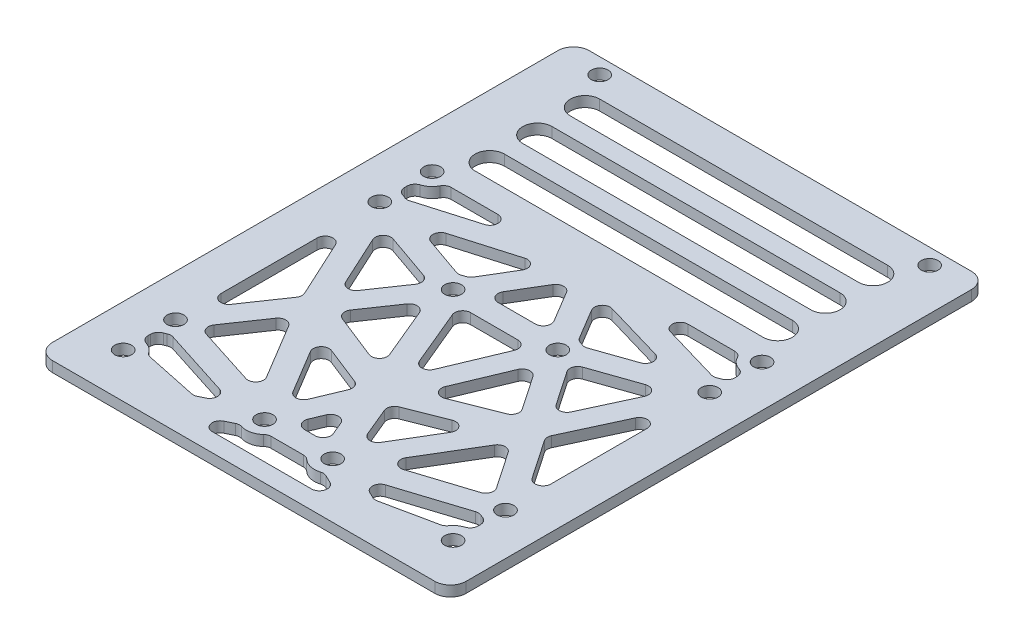
from build123d import *

# Parameters (mm, degrees)
SKETCH_1_W          = 79
SKETCH_1_H          = 102.5
SKETCH_1_R          = 1.6
EXTRUDE_1_DEPTH     = 2
CUT_EXTRUDE_1_DEPTH = 69.558369292
FILLET_R1_5_R       = 1.5
FILLET_R3_R         = 3


with BuildPart() as part:
    # 草图1 → 凸台-拉伸1 (new body)
    with BuildSketch(Plane(origin=(0, 0, 0), x_dir=(1, 0, 0), z_dir=(0, 1, 0))):
        with Locations((0, 4.75)):
            Rectangle(SKETCH_1_W, SKETCH_1_H)
        with Locations(Location((-31.5, 11, 0), (0, 0, 270))):
            Circle(SKETCH_1_R, mode=Mode.SUBTRACT)
        with Locations(Location((-31.5, 21, 0), (0, 0, 270))):
            Circle(SKETCH_1_R, mode=Mode.SUBTRACT)
        with Locations(Location((31.5, 11, 0), (0, 0, 90))):
            Circle(SKETCH_1_R, mode=Mode.SUBTRACT)
        with Locations(Location((31.5, 21, 0), (0, 0, 90))):
            Circle(SKETCH_1_R, mode=Mode.SUBTRACT)
        with Locations(Location((-6.5, -36, 0), (0, 0, 270))):
            Circle(SKETCH_1_R, mode=Mode.SUBTRACT)
        with Locations(Location((6.5, -36, 0), (0, 0, 90))):
            Circle(SKETCH_1_R, mode=Mode.SUBTRACT)
        with Locations(Location((-10, 3.5, 0), (0, 0, 270))):
            Circle(SKETCH_1_R, mode=Mode.SUBTRACT)
        with Locations(Location((10, 3.5, 0), (0, 0, 90))):
            Circle(SKETCH_1_R, mode=Mode.SUBTRACT)
        with Locations(Location((-31.5, 53, 0), (0, 0, 270))):
            Circle(SKETCH_1_R, mode=Mode.SUBTRACT)
        with Locations(Location((31.5, 53, 0), (0, 0, 90))):
            Circle(SKETCH_1_R, mode=Mode.SUBTRACT)
        with Locations(Location((-31.5, -28, 0), (0, 0, 270))):
            Circle(SKETCH_1_R, mode=Mode.SUBTRACT)
        with Locations(Location((-31.5, -38, 0), (0, 0, 270))):
            Circle(SKETCH_1_R, mode=Mode.SUBTRACT)
        with Locations(Location((31.5, -38, 0), (0, 0, 90))):
            Circle(SKETCH_1_R, mode=Mode.SUBTRACT)
        with Locations(Location((31.5, -28, 0), (0, 0, 90))):
            Circle(SKETCH_1_R, mode=Mode.SUBTRACT)
    extrude(amount=EXTRUDE_1_DEPTH)

    # 草图2 → 切除-拉伸1 (cut, through all)
    with BuildSketch(Plane(origin=(0, 2, 0), x_dir=(1, 0, 0), z_dir=(0, 1, 0))):
        with BuildLine():
            Line((-27.5, 43.4), (27.5, 43.4))
            ThreePointArc((27.5, 43.4), (30.3, 46.2), (27.5, 49))
            Line((27.5, 49), (-27.5, 49))
            ThreePointArc((-27.5, 49), (-30.3, 46.2), (-27.5, 43.4))
        make_face()
        with BuildLine():
            Line((-27.5, 34.3), (27.5, 34.3))
            ThreePointArc((27.5, 34.3), (30.3, 37.1), (27.5, 39.9))
            Line((27.5, 39.9), (-27.5, 39.9))
            ThreePointArc((-27.5, 39.9), (-30.3, 37.1), (-27.5, 34.3))
        make_face()
        with BuildLine():
            Line((-27.5, 25.2), (27.5, 25.2))
            ThreePointArc((27.5, 25.2), (30.3, 28), (27.5, 30.8))
            Line((27.5, 30.8), (-27.5, 30.8))
            ThreePointArc((-27.5, 30.8), (-30.3, 28), (-27.5, 25.2))
        make_face()
        with BuildLine():
            Line((-31.5, 17.5), (-31.5, 14.5))
            ThreePointArc((-31.5, 14.5), (-30.423705251, 14.330403821), (-29.451716488, 13.838051207))
            Line((-29.451716488, 13.838051207), (-7.668957034, 20.2))
            Line((-7.668957034, 20.2), (-28.092654993, 20.2))
            ThreePointArc((-28.092654993, 20.2), (-29.326293488, 18.256826655), (-31.5, 17.5))
        make_face()
        with BuildLine():
            ThreePointArc((29.451716488, 13.838051207), (30.423705251, 14.330403821), (31.5, 14.5))
            Line((31.5, 14.5), (31.5, 17.5))
            ThreePointArc((31.5, 17.5), (29.326293488, 18.256826655), (28.092654993, 20.2))
            Line((28.092654993, 20.2), (7.668957034, 20.2))
            Line((7.668957034, 20.2), (29.451716488, 13.838051207))
        make_face()
        with BuildLine():
            Line((-24.452290628, 10.818556238), (-11.899535217, 6.439688072))
            ThreePointArc((-11.899535217, 6.439688072), (-11.192938065, 6.790425318), (-10.425740034, 6.974009992))
            Line((-10.425740034, 6.974009992), (-4.662637344, 16.598391483))
            Line((-4.662637344, 16.598391483), (-24.452290628, 10.818556238))
        make_face()
        Polygon((-6.206589312, 5.65), (6.206589312, 5.65), (0, 16.015004152), align=None)
        with BuildLine():
            Line((11.899535217, 6.439688072), (24.452290628, 10.818556238))
            Line((24.452290628, 10.818556238), (4.662637344, 16.598391483))
            Line((4.662637344, 16.598391483), (10.425740034, 6.974009992))
            ThreePointArc((10.425740034, 6.974009992), (11.192938065, 6.790425318), (11.899535217, 6.439688072))
        make_face()
        Polygon((-27.420486956, 7.299854547), (-20.389131694, -7.907495205), (-13.357776432, 2.394257853), align=None)
        Polygon((-17.456513392, -11.238449922), (-3.946122396, -16.570590362), (-10.457154201, -0.983574828), align=None)
        Polygon((-6.771858845, 1.35), (0, -14.86141966), (6.771858845, 1.35), align=None)
        Polygon((-31.5, 5.87701259), (-31.5, -24.186209235), (-23.213342702, -12.045292729), align=None)
        Polygon((13.357776432, 2.394257853), (20.389131694, -7.907495205), (27.420486956, 7.299854547), align=None)
        Polygon((10.457154201, -0.983574828), (3.946122396, -16.570590362), (17.456513392, -11.238449922), align=None)
        Polygon((23.213342702, -12.045292729), (31.5, -24.186209235), (31.5, 5.87701259), align=None)
        Polygon((-28.098995565, -26.830923802), (-11.279390947, -32.21319728), (-20.866565579, -16.234572893), align=None)
        Polygon((-15.647599969, -16.575151194), (-6.844560738, -31.246883245), (-2.829139335, -21.634207764), align=None)
        Polygon((-3.271858845, -33.85), (3.271858845, -33.85), (0, -26.017368219), align=None)
        Polygon((2.829139335, -21.634207764), (6.844560738, -31.246883245), (15.647599969, -16.575151194), align=None)
        Polygon((20.866565579, -16.234572893), (11.279390947, -32.21319728), (28.098995565, -26.830923802), align=None)
        with BuildLine():
            Line((-28.354506597, -36.465115232), (-17.21554823, -38.810303281))
            Line((-17.21554823, -38.810303281), (-12.270862978, -36.410721464))
            Line((-12.270862978, -36.410721464), (-29.52486957, -30.889439354))
            ThreePointArc((-29.52486957, -30.889439354), (-30.466326391, -31.343877819), (-31.5, -31.5))
            Line((-31.5, -31.5), (-31.5, -34.5))
            ThreePointArc((-31.5, -34.5), (-29.645558937, -35.031658991), (-28.354506597, -36.465115232))
        make_face()
        with BuildLine():
            Line((-8.046002547, -39.140043969), (-16, -43))
            Line((-16, -43), (16, -43))
            Line((16, -43), (8.046002547, -39.140043969))
            ThreePointArc((8.046002547, -39.140043969), (5.716046361, -39.41107266), (3.738207104, -38.15))
            Line((3.738207104, -38.15), (-3.738207104, -38.15))
            ThreePointArc((-3.738207104, -38.15), (-5.716046361, -39.41107266), (-8.046002547, -39.140043969))
        make_face()
        with BuildLine():
            Line((12.270862978, -36.410721464), (17.21554823, -38.810303281))
            Line((17.21554823, -38.810303281), (28.354506597, -36.465115232))
            ThreePointArc((28.354506597, -36.465115232), (29.645558937, -35.031658991), (31.5, -34.5))
            Line((31.5, -34.5), (31.5, -31.5))
            ThreePointArc((31.5, -31.5), (30.466326391, -31.343877819), (29.52486957, -30.889439354))
            Line((29.52486957, -30.889439354), (12.270862978, -36.410721464))
        make_face()
    extrude(amount=-CUT_EXTRUDE_1_DEPTH, mode=Mode.SUBTRACT)

    # R1.5 镂空圆角
    fillet_r1_5_edges = [part.edges().sort_by_distance(p)[0] for p in [
        (-28.354506597, 1, 36.465115232),
        (-31.5, 1, 34.5),
        (-31.5, 1, 31.5),
        (-29.52486957, 1, 30.889439354),
        (-12.270862978, 1, 36.410721464),
        (-17.21554823, 1, 38.810303281),
        (28.098995565, 1, 26.830923802),
        (11.279390947, 1, 32.21319728),
        (20.866565579, 1, 16.234572893),
        (-3.271858845, 1, 33.85),
        (0, 1, 26.017368219),
        (3.271858845, 1, 33.85),
        (15.647599969, 1, 16.575151194),
        (6.844560738, 1, 31.246883245),
        (2.829139335, 1, 21.634207764),
        (28.354506597, 1, 36.465115232),
        (17.21554823, 1, 38.810303281),
        (12.270862978, 1, 36.410721464),
        (29.52486957, 1, 30.889439354),
        (31.5, 1, 31.5),
        (31.5, 1, 34.5),
        (8.046002547, 1, 39.140043969),
        (16, 1, 43),
        (-16, 1, 43),
        (-8.046002547, 1, 39.140043969),
        (-3.738207104, 1, 38.15),
        (3.738207104, 1, 38.15),
        (6.206589312, 1, -5.65),
        (-6.206589312, 1, -5.65),
        (0, 1, -16.015004152),
        (-10.425740034, 1, -6.974009992),
        (-11.899535217, 1, -6.439688072),
        (-24.452290628, 1, -10.818556238),
        (-4.662637344, 1, -16.598391483),
        (10.425740034, 1, -6.974009992),
        (4.662637344, 1, -16.598391483),
        (24.452290628, 1, -10.818556238),
        (11.899535217, 1, -6.439688072),
        (-27.420486956, 1, -7.299854547),
        (-13.357776432, 1, -2.394257853),
        (-20.389131694, 1, 7.907495205),
        (28.092654993, 1, -20.2),
        (31.5, 1, -17.5),
        (31.5, 1, -14.5),
        (29.451716488, 1, -13.838051207),
        (7.668957034, 1, -20.2),
        (-31.5, 1, -17.5),
        (-28.092654993, 1, -20.2),
        (-7.668957034, 1, -20.2),
        (-29.451716488, 1, -13.838051207),
        (-31.5, 1, -14.5),
        (-20.866565579, 1, 16.234572893),
        (-11.279390947, 1, 32.21319728),
        (-28.098995565, 1, 26.830923802),
        (-15.647599969, 1, 16.575151194),
        (-2.829139335, 1, 21.634207764),
        (-6.844560738, 1, 31.246883245),
        (31.5, 1, -5.87701259),
        (31.5, 1, 24.186209235),
        (23.213342702, 1, 12.045292729),
        (17.456513392, 1, 11.238449922),
        (3.946122396, 1, 16.570590362),
        (10.457154201, 1, 0.983574828),
        (0, 1, 14.86141966),
        (-6.771858845, 1, -1.35),
        (6.771858845, 1, -1.35),
        (-17.456513392, 1, 11.238449922),
        (-10.457154201, 1, 0.983574828),
        (-3.946122396, 1, 16.570590362),
        (-31.5, 1, -5.87701259),
        (-23.213342702, 1, 12.045292729),
        (-31.5, 1, 24.186209235),
        (27.420486956, 1, -7.299854547),
        (20.389131694, 1, 7.907495205),
        (13.357776432, 1, -2.394257853),
    ]]
    fillet(fillet_r1_5_edges, radius=FILLET_R1_5_R)

    # R3 外缘圆角
    fillet_r3_edges = [part.edges().sort_by_distance(p)[0] for p in [
        (-39.5, 1, -56),
        (39.5, 1, -56),
        (39.5, 1, 46.5),
        (-39.5, 1, 46.5),
    ]]
    fillet(fillet_r3_edges, radius=FILLET_R3_R)


solid = part.part
